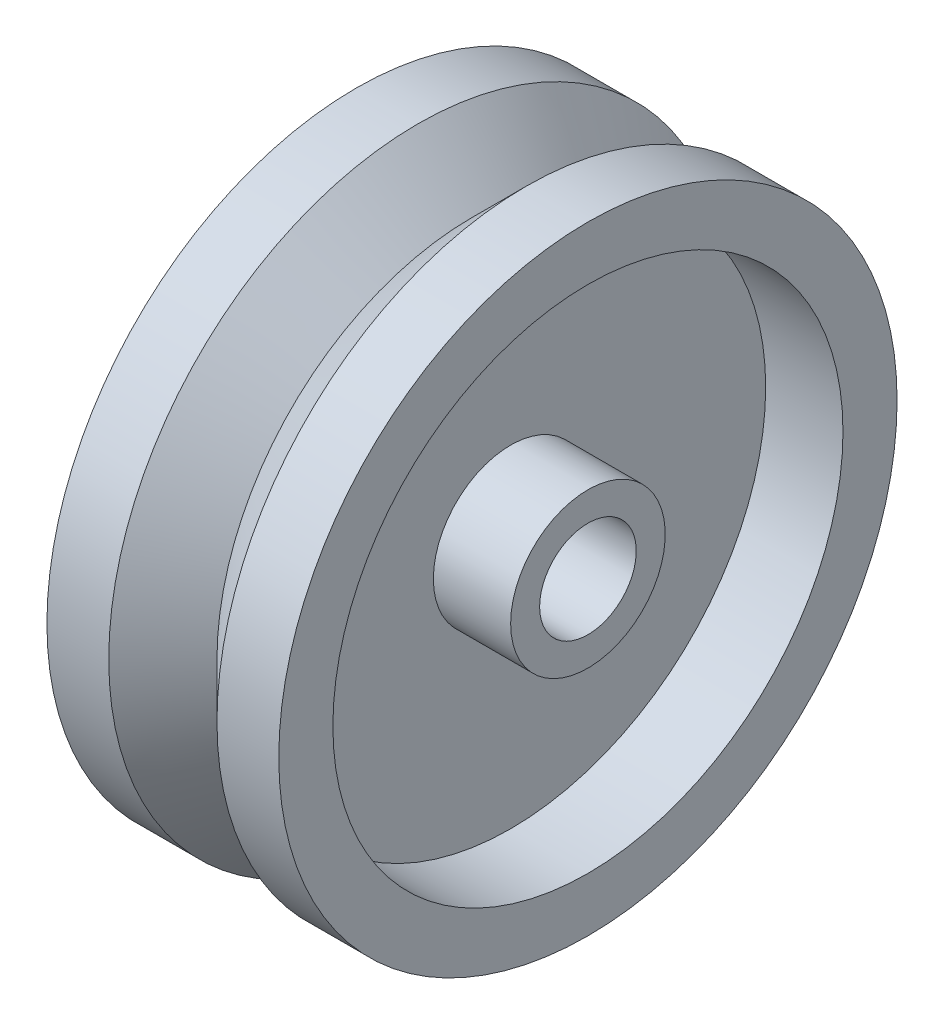
SolidWorks part; units mm, degrees
ref_plane "Front Plane" through (0, 0, 0) normal (0, 0, 1) x (1, 0, 0)
ref_plane "Top Plane" through (0, 0, 0) normal (0, 1, 0) x (1, 0, 0)
ref_plane "Right Plane" through (0, 0, 0) normal (1, 0, 0) x (0, 0, -1)
sketch "Sketch1" plane through (0, 0, 0) normal (0, 0, 1) x (1, 0, 0)
  line L0 (-45.5, 0) -> (54, 0) construction
  line L1 (0, 54.125) -> (0, -45.875) construction
  line L2 (3.5, 20) -> (0, 16.5)
  line L3 (-3.5, 20) -> (-7.5, 20)
  line L4 (-7.5, 20) -> (-7.5, 16.5)
  line L5 (-7.5, 16.5) -> (-2.5, 16.5)
  line L6 (-2.5, 16.5) -> (-2.5, 5)
  line L7 (-2.5, 5) -> (-7.5, 5)
  line L8 (-7.5, 5) -> (-7.5, 3.125)
  line L9 (-7.5, 3.125) -> (7.5, 3.125)
  line L10 (7.5, 3.125) -> (7.5, 5)
  line L11 (7.5, 5) -> (2.5, 5)
  line L12 (2.5, 5) -> (2.5, 16.5)
  line L13 (2.5, 16.5) -> (7.5, 16.5)
  line L14 (7.5, 16.5) -> (7.5, 20)
  line L15 (7.5, 20) -> (3.5, 20)
  line L16 (0, 16.5) -> (-3.5, 20)
  dimension "D1" = 2.5
  dimension "D2" = 5
  dimension "D3" = 15
  dimension "D4" = 7.5
  dimension "D5" = 7.5
  dimension "D6" = 4
  dimension "D7" = 4
  dimension "D8" = 15
  dimension "D9" = 3.125
  dimension "D10" = 5
  dimension "D11" = 16.5
  dimension "D12" = 16.5
  dimension "D13" = 20
  dimension "D14" = 90
  dimension "D15" = 20
revolve "Revolve1" add sketch "Sketch1" angle 360 about L0
